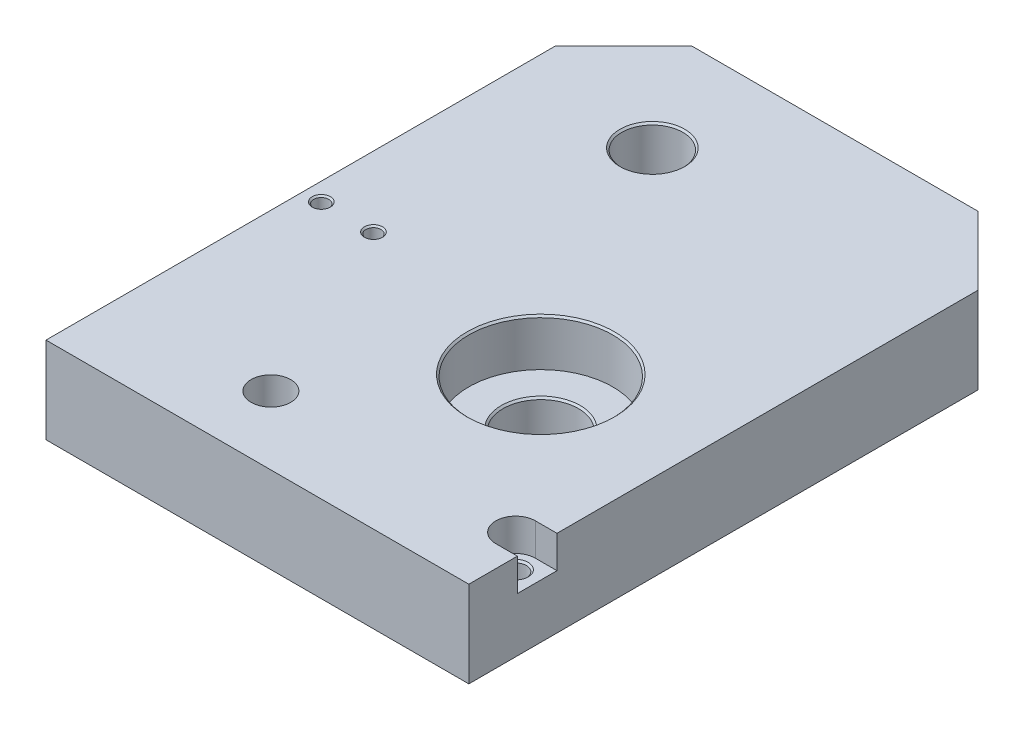
from build123d import *

# Parameters (mm, degrees)
BOSS_EXTRUDE1_DEPTH         = 24
SKETCH_2_2_R                = 8.5
SKETCH_2_2_R_2              = 20
SKETCH_2_2_R_3              = 3
CUT_EXTRUDE1_DEPTH          = 13
SKETCH_2_2_2_R              = 8.5
SKETCH_2_2_2_R_2            = 3
CUT_EXTRUDE2_DEPTH          = 103.311411876
SKETCH3_R                   = 10.5
CUT_EXTRUDE3_DEPTH          = 101.302666964
M5_TAPPED_HOLE1_D           = 4.2
M5_TAPPED_HOLE1_CSINK_D     = 5.05
M5_TAPPED_HOLE1_CSINK_ANGLE = 90
CHAMFER1_SIZE               = 0.5
CUT_EXTRUDE4_START          = -24
SKETCH6_R                   = 5.5
SKETCH6_R_2                 = 3
SKETCH6_W                   = 5.693229178
SKETCH6_H                   = 11
CUT_EXTRUDE4_DEPTH          = 9
CHAMFER2_SIZE               = 0.5


with BuildPart() as part:
    # Sketch1 → Boss-Extrude1 (new body)
    with BuildSketch(Plane(origin=(0, 0, 0), x_dir=(1, 0, 0), z_dir=(0, 1, 0))):
        Polygon((-58.75, 61.25), (-39.75, 80.25), (39.75, 80.25), (58.75, 61.25), (58.75, -80.25), (-58.75, -80.25), align=None)
    extrude(amount=BOSS_EXTRUDE1_DEPTH)

    # Sketch 2_2 → Cut-Extrude1 (cut)
    with BuildSketch(Plane(origin=(0, 24, 0), x_dir=(1, 0, 0), z_dir=(0, 1, 0))):
        with Locations(Location((-20.75, 50.25, 0), (0, 0, 270))):
            Circle(SKETCH_2_2_R)
        with Locations(Location((18.25, -19.75, 0), (0, 0, 270))):
            Circle(SKETCH_2_2_R_2)
        with Locations(Location((52.75, -61.25, 0), (0, 0, 270))):
            Circle(SKETCH_2_2_R_3)
        with Locations(Location((-15.25, -61.25, 0), (0, 0, 270))):
            Circle(SKETCH_2_2_R_3)
    extrude(amount=-CUT_EXTRUDE1_DEPTH, mode=Mode.SUBTRACT)

    # Sketch 2_2 2 → Cut-Extrude2 (cut, through all)
    with BuildSketch(Plane(origin=(0, 24, 0), x_dir=(1, 0, 0), z_dir=(0, 1, 0))):
        with Locations(Location((-20.75, 50.25, 0), (0, 0, 270))):
            Circle(SKETCH_2_2_2_R)
        with Locations(Location((52.75, -61.25, 0), (0, 0, 270))):
            Circle(SKETCH_2_2_2_R_2)
        with Locations(Location((-15.25, -61.25, 0), (0, 0, 270))):
            Circle(SKETCH_2_2_2_R_2)
    extrude(amount=-CUT_EXTRUDE2_DEPTH, mode=Mode.SUBTRACT)

    # Sketch3 → Cut-Extrude3 (cut, through all)
    with BuildSketch(Plane(origin=(0, 11, 0), x_dir=(1, 0, 0), z_dir=(0, 1, 0))):
        with Locations(Location((18.25, -19.75, 0), (0, 0, 270))):
            Circle(SKETCH3_R)
    extrude(amount=-CUT_EXTRUDE3_DEPTH, mode=Mode.SUBTRACT)

    # M5 Tapped Hole1 (through all)
    with Locations(Plane(origin=(0, 24, 0), x_dir=(1, 0, 0), z_dir=(0, 1, 0))):
        with Locations((-39.25, -8.75), (-53.75, -8.75)):
            CounterSinkHole(M5_TAPPED_HOLE1_D / 2, M5_TAPPED_HOLE1_CSINK_D / 2, counter_sink_angle=M5_TAPPED_HOLE1_CSINK_ANGLE)

    # Chamfer1
    chamfer1_edges = [part.edges().sort_by_distance(p)[0] for p in [
        (-20.75, 24, -58.75),
        (18.25, 24, -0.25),
        (-20.75, 0, -58.75),
        (18.25, 11, 9.25),
    ]]
    chamfer(chamfer1_edges, length=CHAMFER1_SIZE)

    # Sketch6 → Cut-Extrude4 (cut)
    # profile 1 of 7: a face of its own
    with BuildSketch(Plane.XZ.offset(CUT_EXTRUDE4_START)):
        with Locations(Location((-15.25, 61.25, 0), (0, 0, 90))):
            Circle(SKETCH6_R)
        with Locations(Location((-15.25, 61.25, 0), (0, 0, 90))):
            Circle(SKETCH6_R_2, mode=Mode.SUBTRACT)
    # profile 2 of 7: a face of its own
    with BuildSketch(Plane.XZ.offset(CUT_EXTRUDE4_START)):
        with BuildLine():
            ThreePointArc((58.25, 61.25), (56.639087297, 65.139087297), (52.75, 66.75))
            ThreePointArc((52.75, 66.75), (52.40269227, 66.73902335), (52.056770822, 66.706137215))
            Line((52.056770822, 66.706137215), (52.056770822, 64.168806829))
            ThreePointArc((52.056770822, 64.168806829), (54.610149519, 63.603687271), (55.75, 61.25))
            ThreePointArc((55.75, 61.25), (54.610149519, 58.896312729), (52.056770822, 58.331193171))
            Line((52.056770822, 58.331193171), (52.056770822, 55.793862785))
            ThreePointArc((52.056770822, 55.793862785), (52.40269227, 55.76097665), (52.75, 55.75))
            ThreePointArc((52.75, 55.75), (56.639087297, 57.360912703), (58.25, 61.25))
        make_face()
    # profile 3 of 7: a face of its own
    with BuildSketch(Plane.XZ.offset(CUT_EXTRUDE4_START)):
        with BuildLine():
            Line((52.056770822, 64.168806829), (52.056770822, 66.706137215))
            ThreePointArc((52.056770822, 66.706137215), (47.25, 61.25), (52.056770822, 55.793862785))
            Line((52.056770822, 55.793862785), (52.056770822, 58.331193171))
            ThreePointArc((52.056770822, 58.331193171), (49.75, 61.25), (52.056770822, 64.168806829))
        make_face()
    # profile 4 of 7: a face of its own
    with BuildSketch(Plane.XZ.offset(CUT_EXTRUDE4_START)):
        with Locations((61.596614589, 61.25)):
            Rectangle(SKETCH6_W, SKETCH6_H)
    # profile 5 of 7: a face of its own
    with BuildSketch(Plane.XZ.offset(CUT_EXTRUDE4_START)):
        with BuildLine():
            ThreePointArc((58.25, 61.25), (56.639087297, 65.139087297), (52.75, 66.75))
            ThreePointArc((52.75, 66.75), (52.40269227, 66.73902335), (52.056770822, 66.706137215))
            Line((52.056770822, 66.706137215), (52.056770822, 64.168806829))
            ThreePointArc((52.056770822, 64.168806829), (54.610149519, 63.603687271), (55.75, 61.25))
            ThreePointArc((55.75, 61.25), (54.610149519, 58.896312729), (52.056770822, 58.331193171))
            Line((52.056770822, 58.331193171), (52.056770822, 55.793862785))
            ThreePointArc((52.056770822, 55.793862785), (52.40269227, 55.76097665), (52.75, 55.75))
            ThreePointArc((52.75, 55.75), (56.639087297, 57.360912703), (58.25, 61.25))
        make_face()
    # profile 6 of 7: a face of its own
    with BuildSketch(Plane.XZ.offset(CUT_EXTRUDE4_START)):
        with BuildLine():
            Line((52.056770822, 64.168806829), (52.056770822, 66.706137215))
            ThreePointArc((52.056770822, 66.706137215), (47.25, 61.25), (52.056770822, 55.793862785))
            Line((52.056770822, 55.793862785), (52.056770822, 58.331193171))
            ThreePointArc((52.056770822, 58.331193171), (49.75, 61.25), (52.056770822, 64.168806829))
        make_face()
    # profile 7 of 7: a face of its own
    with BuildSketch(Plane.XZ.offset(CUT_EXTRUDE4_START)):
        with BuildLine():
            Line((58.75, 66.75), (52.75, 66.75))
            ThreePointArc((52.75, 66.75), (56.639087297, 65.139087297), (58.25, 61.25))
            ThreePointArc((58.25, 61.25), (56.639087297, 57.360912703), (52.75, 55.75))
            Line((52.75, 55.75), (58.75, 55.75))
            Line((58.75, 55.75), (58.75, 66.75))
        make_face()
    extrude(amount=CUT_EXTRUDE4_DEPTH, mode=Mode.SUBTRACT)

    # Chamfer2
    chamfer2_edges = [part.edges().sort_by_distance(p)[0] for p in [
        (52.75, 15, 58.25),
    ]]
    chamfer(chamfer2_edges, length=CHAMFER2_SIZE)


solid = part.part
